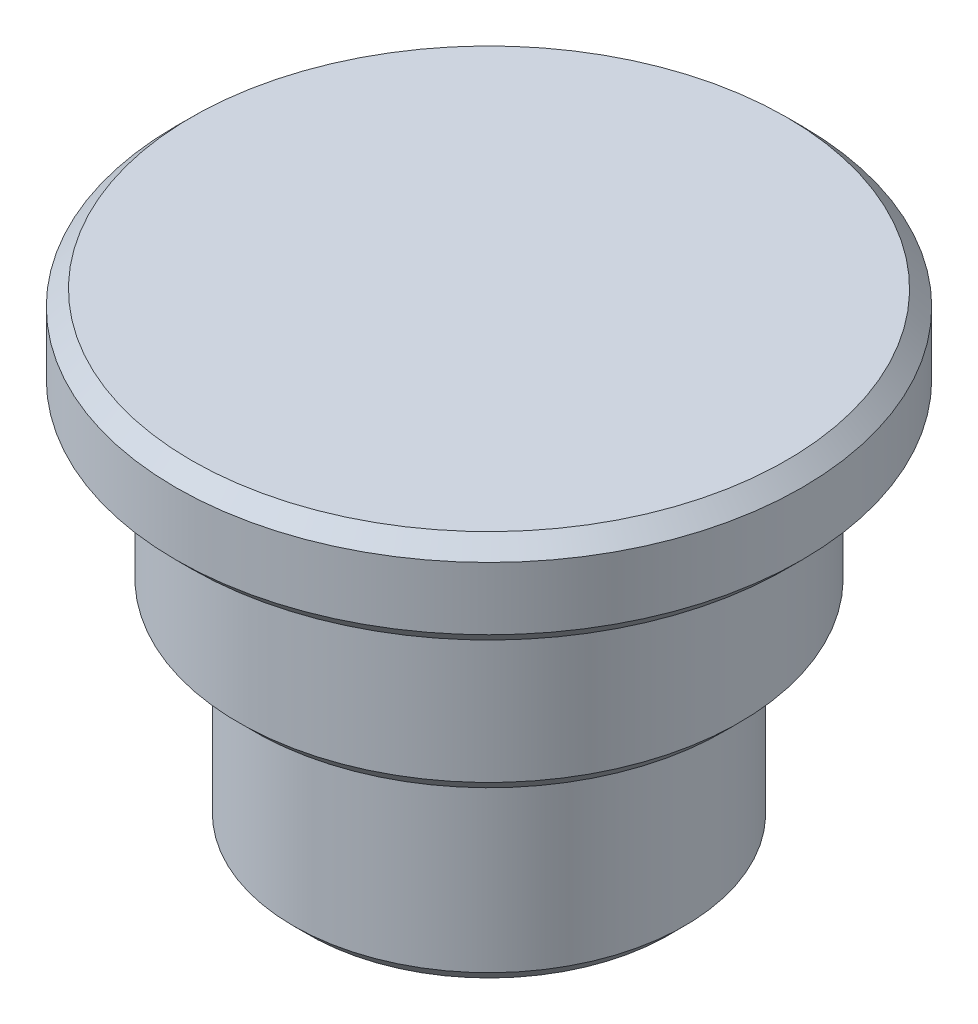
SolidWorks part; units mm, degrees
material "Q235B"
ref_plane "Front Plane" through (0, 0, 0) normal (0, 0, 1) x (1, 0, 0)
ref_plane "Top Plane" through (0, 0, 0) normal (0, 1, 0) x (1, 0, 0)
ref_plane "Right Plane" through (0, 0, 0) normal (1, 0, 0) x (0, 0, -1)
sketch "Sketch1" plane through (0, 0, 0) normal (0, 0, 1) x (1, 0, 0)
  line L0 (82.463, -48.25) -> (82.463, -36.25) construction
  line L1 (92.463, -48.25) -> (31.463, -48.25) construction
  line L2 (-172.537, -36.25) -> (107.463, -36.25) construction
  line L3 (88.713, -48.25) -> (88.713, -42.25) construction
  line L4 (88.713, -48.25) -> (88.713, -41.75)
  line L5 (88.713, -41.75) -> (90.463, -41.75)
  line L6 (90.463, -42.25) -> (90.463, -36.25) construction
  line L7 (90.463, -41.75) -> (90.463, -36.25)
  line L8 (90.463, -36.25) -> (92.463, -36.25)
  line L9 (92.463, -36.25) -> (92.463, -33.25)
  line L10 (92.463, -33.25) -> (82.463, -33.25)
  line L11 (82.463, -36.25) -> (82.463, -33.25) construction
  line L12 (88.713, -48.25) -> (82.463, -48.25)
  line L13 (82.463, -48.25) -> (82.463, -33.25)
  dimension "D1" = 6.25
  dimension "D2" = 3
  dimension "D3" = 20
  dimension "D4" = 5.5
revolve "Revolve1" add sketch "Sketch1" angle 360 about L13
chamfer "Chamfer1" distance 0.5 angle 45 4 edges at (82.463, -48.25, -6.25) (82.463, -41.75, -8) (82.463, -36.25, -10) (82.463, -33.25, -10)
